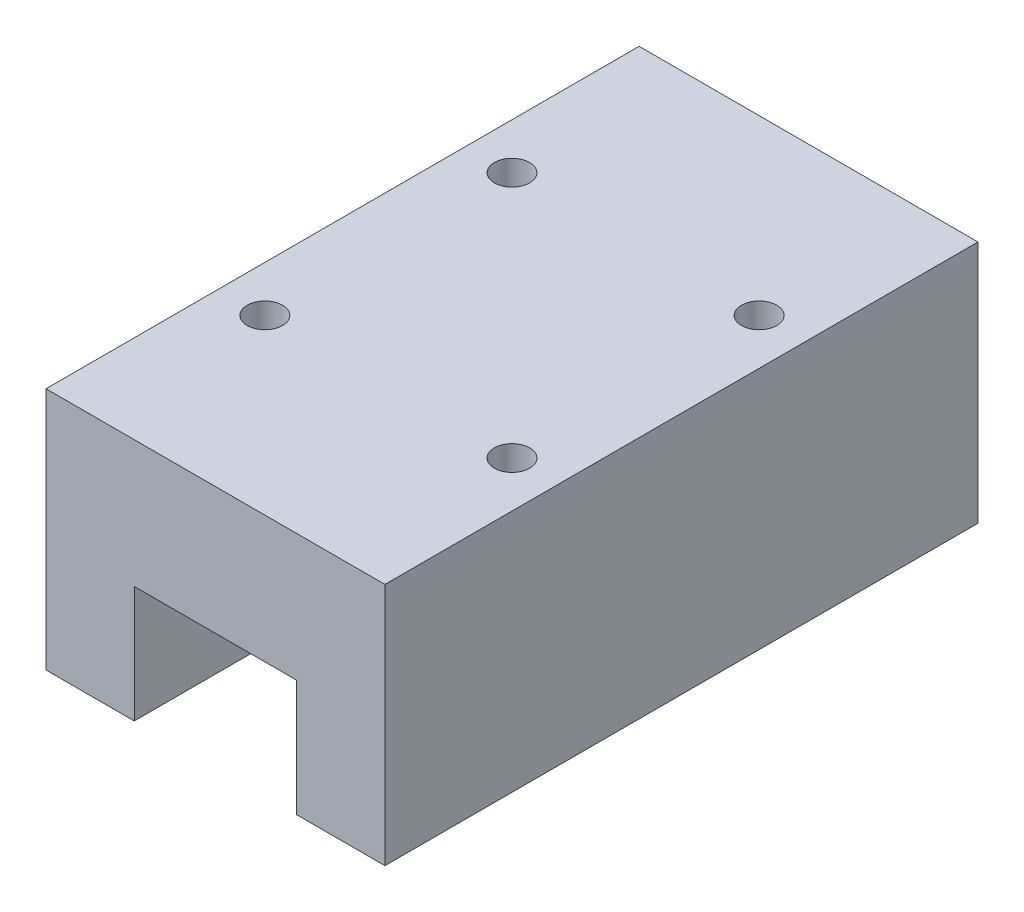
from build123d import *

# Parameters (mm, degrees)
EXTRUDE_1_DEPTH        = 42
HOLE_WIZARD_M6_1_D     = 5
HOLE_WIZARD_M6_1_DEPTH = 8
HOLE_WIZARD_M6_1_TIP   = 1.502151548


with BuildPart() as part:
    # 草图1 → 凸台-拉伸1 (new, symmetric)
    with BuildSketch(Plane.XY):
        Polygon((-11.5, -17.25), (-24, -17.25), (-24, 17.25), (24, 17.25), (24, -17.25), (11.5, -17.25), (11.5, -0.75), (-11.5, -0.75), align=None)
    extrude(amount=EXTRUDE_1_DEPTH, both=True)

    # M6 螺纹孔1
    with Locations(Plane(origin=(0, 17.25, 0), x_dir=(1, 0, 0), z_dir=(0, 1, 0))):
        with Locations((-17.5, 17.5), (17.5, 17.5), (17.5, -17.5), (-17.5, -17.5)):
            Hole(HOLE_WIZARD_M6_1_D / 2, depth=HOLE_WIZARD_M6_1_DEPTH)
            with Locations((0, 0, -(HOLE_WIZARD_M6_1_DEPTH + HOLE_WIZARD_M6_1_TIP / 2))):  # 118° drill point
                Cone(0, HOLE_WIZARD_M6_1_D / 2, HOLE_WIZARD_M6_1_TIP, mode=Mode.SUBTRACT)


solid = part.part
